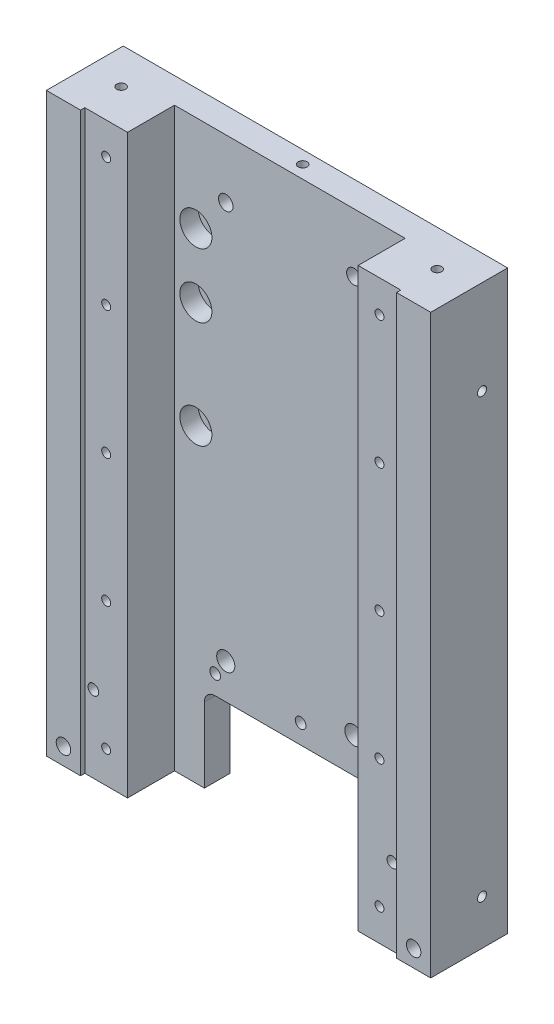
from build123d import *

# Parameters (mm, degrees)
SKETCH_1_W                     = 180
SKETCH_1_H                     = 270
EXTRUDE_1_DEPTH                = 34
SKETCH_2_W                     = 108
SKETCH_2_H                     = 22
CUT_EXTRUDE_1_DEPTH            = 287.628679654
SKETCH_3_W                     = 16
SKETCH_3_H                     = 270
EXTRUDE_2_DEPTH                = 2
HOLE_WIZARD_M8_1_D             = 6.8
HOLE_WIZARD_M8_1_DEPTH         = 19.75
HOLE_WIZARD_M8_1_TIP           = 2.042926105
SKETCH_6_W                     = 80
SKETCH_6_H                     = 40
CUT_EXTRUDE_2_DEPTH            = 165.015243194
FILLET_1_R                     = 5
HOLE_WIZARD_M5_1_D             = 4.2
HOLE_WIZARD_M5_1_DEPTH         = 12.4
HOLE_WIZARD_M5_1_TIP           = 1.2618073
HOLE_WIZARD_M6_1_D             = 5
HOLE_WIZARD_M6_1_DEPTH         = 15
HOLE_WIZARD_M6_1_TIP           = 1.502151548
HOLE_WIZARD_M8_2_D             = 6.8
HOLE_WIZARD_M10_1_D            = 8.5
HOLE_WIZARD_M8_1_2_D           = 9
HOLE_WIZARD_M8_1_2_CBORE_D     = 15
HOLE_WIZARD_M8_1_2_CBORE_DEPTH = 8.6
HOLE_WIZARD_M5_3_D             = 4.2
HOLE_WIZARD_M5_3_DEPTH         = 12.4
HOLE_WIZARD_M5_3_TIP           = 1.2618073
HOLE_WIZARD_M5_4_D             = 4.2
HOLE_WIZARD_M5_4_DEPTH         = 12.4
HOLE_WIZARD_M5_4_TIP           = 1.2618073
HOLE_WIZARD_M6_2_D             = 5
HOLE_WIZARD_M4_1_D             = 3.3
HOLE_WIZARD_M4_1_DEPTH         = 10.1
HOLE_WIZARD_M4_1_TIP           = 0.991420021
HOLE_WIZARD_M5_5_D             = 4.2
HOLE_WIZARD_M5_5_DEPTH         = 12.4
HOLE_WIZARD_M5_5_TIP           = 1.2618073


with BuildPart() as part:
    # 草图1 → 凸台-拉伸1 (new body)
    with BuildSketch(Plane.XY):
        Rectangle(SKETCH_1_W, SKETCH_1_H)
    extrude(amount=EXTRUDE_1_DEPTH)

    # 草图2 → 切除-拉伸1 (cut, through all)
    with BuildSketch(Plane.XZ.offset(135)):
        with Locations((0, 23)):
            Rectangle(SKETCH_2_W, SKETCH_2_H)
    extrude(amount=-CUT_EXTRUDE_1_DEPTH, mode=Mode.SUBTRACT)

    # 草图3 → 凸台-拉伸2 (add)
    with BuildSketch(Plane.XY.offset(34)):
        with Locations((-82, 0)):
            Rectangle(SKETCH_3_W, SKETCH_3_H)
        with Locations((82, 0)):
            Rectangle(SKETCH_3_W, SKETCH_3_H)
    extrude(amount=EXTRUDE_2_DEPTH)

    # Hole Wizard M8 _1
    with Locations(Plane.XY.offset(36)):
        with Locations((-82, -127), (82, -127)):
            Hole(HOLE_WIZARD_M8_1_D / 2, depth=HOLE_WIZARD_M8_1_DEPTH)
            with Locations((0, 0, -(HOLE_WIZARD_M8_1_DEPTH + HOLE_WIZARD_M8_1_TIP / 2))):  # 118° drill point
                Cone(0, HOLE_WIZARD_M8_1_D / 2, HOLE_WIZARD_M8_1_TIP, mode=Mode.SUBTRACT)

    # 草图6 → 切除-拉伸2 (cut, through all)
    with BuildSketch(Plane.XY.offset(12)):
        with Locations((0, -115)):
            Rectangle(SKETCH_6_W, SKETCH_6_H)
    extrude(amount=-CUT_EXTRUDE_2_DEPTH, mode=Mode.SUBTRACT)

    # 圆角1
    fillet_1_edges = [part.edges().sort_by_distance(p)[0] for p in [
        (40, -95, 6),
        (-40, -95, 6),
    ]]
    fillet(fillet_1_edges, radius=FILLET_1_R)

    # M5 螺纹孔1
    with Locations(Plane(origin=(0, 135, 0), x_dir=(1, 0, 0), z_dir=(0, 1, 0))):
        with Locations((-74, -17), (74, -17), (0, -6)):
            Hole(HOLE_WIZARD_M5_1_D / 2, depth=HOLE_WIZARD_M5_1_DEPTH)
            with Locations((0, 0, -(HOLE_WIZARD_M5_1_DEPTH + HOLE_WIZARD_M5_1_TIP / 2))):  # 118° drill point
                Cone(0, HOLE_WIZARD_M5_1_D / 2, HOLE_WIZARD_M5_1_TIP, mode=Mode.SUBTRACT)

    # M6 螺纹孔1
    with Locations(Plane(origin=(0, 0, 0), x_dir=(-1, 0, 0), z_dir=(0, 0, -1))):
        with Locations((-45.042166393, -86), (-5.042166393, -86), (34.957833607, -86)):
            Hole(HOLE_WIZARD_M6_1_D / 2, depth=HOLE_WIZARD_M6_1_DEPTH)
            with Locations((0, 0, -(HOLE_WIZARD_M6_1_DEPTH + HOLE_WIZARD_M6_1_TIP / 2))):  # 118° drill point
                Cone(0, HOLE_WIZARD_M6_1_D / 2, HOLE_WIZARD_M6_1_TIP, mode=Mode.SUBTRACT)

    # M8 螺纹孔2 (through all)
    with Locations(Plane.XY.offset(12)):
        with Locations((-30, 107.5), (30, 107.5)):
            Hole(HOLE_WIZARD_M8_2_D / 2)

    # M10 螺纹孔1 (through all)
    with Locations(Plane.XY.offset(12)):
        with Locations((-30, -78.5), (30, -78.5)):
            Hole(HOLE_WIZARD_M10_1_D / 2)

    # Hole Wizard M8 _1 2 (through all)
    with Locations(Plane.XY.offset(12)):
        with Locations((-44, 90.038874186), (-44, 10), (-44, 60), (44, 60), (44, 10), (44, 90.038874186)):
            CounterBoreHole(HOLE_WIZARD_M8_1_2_D / 2, HOLE_WIZARD_M8_1_2_CBORE_D / 2, HOLE_WIZARD_M8_1_2_CBORE_DEPTH)

    # M5 螺纹孔3
    with Locations(Plane.ZY.offset(90)):
        with Locations((12, 91), (12, -114)):
            Hole(HOLE_WIZARD_M5_3_D / 2, depth=HOLE_WIZARD_M5_3_DEPTH)
            with Locations((0, 0, -(HOLE_WIZARD_M5_3_DEPTH + HOLE_WIZARD_M5_3_TIP / 2))):  # 118° drill point
                Cone(0, HOLE_WIZARD_M5_3_D / 2, HOLE_WIZARD_M5_3_TIP, mode=Mode.SUBTRACT)

    # M5 螺纹孔4
    with Locations(Plane(origin=(90, 0, 0), x_dir=(0, 0, -1), z_dir=(1, 0, 0))):
        with Locations((-12, 91), (-12, -114)):
            Hole(HOLE_WIZARD_M5_4_D / 2, depth=HOLE_WIZARD_M5_4_DEPTH)
            with Locations((0, 0, -(HOLE_WIZARD_M5_4_DEPTH + HOLE_WIZARD_M5_4_TIP / 2))):  # 118° drill point
                Cone(0, HOLE_WIZARD_M5_4_D / 2, HOLE_WIZARD_M5_4_TIP, mode=Mode.SUBTRACT)

    # M6 螺纹孔2 (through all)
    with Locations(Plane(origin=(0, 0, 0), x_dir=(-1, 0, 0), z_dir=(0, 0, -1))):
        with Locations((-70, -99), (70, -99)):
            Hole(HOLE_WIZARD_M6_2_D / 2)

    # M4 螺纹孔1
    with Locations(Plane(origin=(0, 0, 0), x_dir=(-1, 0, 0), z_dir=(0, 0, -1))):
        with Locations((-87, 32), (-87, -47), (-87, -126), (87, -126), (87, -47), (87, 32)):
            Hole(HOLE_WIZARD_M4_1_D / 2, depth=HOLE_WIZARD_M4_1_DEPTH)
            with Locations((0, 0, -(HOLE_WIZARD_M4_1_DEPTH + HOLE_WIZARD_M4_1_TIP / 2))):  # 118° drill point
                Cone(0, HOLE_WIZARD_M4_1_D / 2, HOLE_WIZARD_M4_1_TIP, mode=Mode.SUBTRACT)

    # M5 螺纹孔5
    with Locations(Plane.XY.offset(34)):
        with Locations((-64, 0), (-64, 60), (-64, 120), (-64, -120), (-64, -60), (64, -60), (64, -120), (64, 120), (64, 60), (64, 0)):
            Hole(HOLE_WIZARD_M5_5_D / 2, depth=HOLE_WIZARD_M5_5_DEPTH)
            with Locations((0, 0, -(HOLE_WIZARD_M5_5_DEPTH + HOLE_WIZARD_M5_5_TIP / 2))):  # 118° drill point
                Cone(0, HOLE_WIZARD_M5_5_D / 2, HOLE_WIZARD_M5_5_TIP, mode=Mode.SUBTRACT)


solid = part.part
